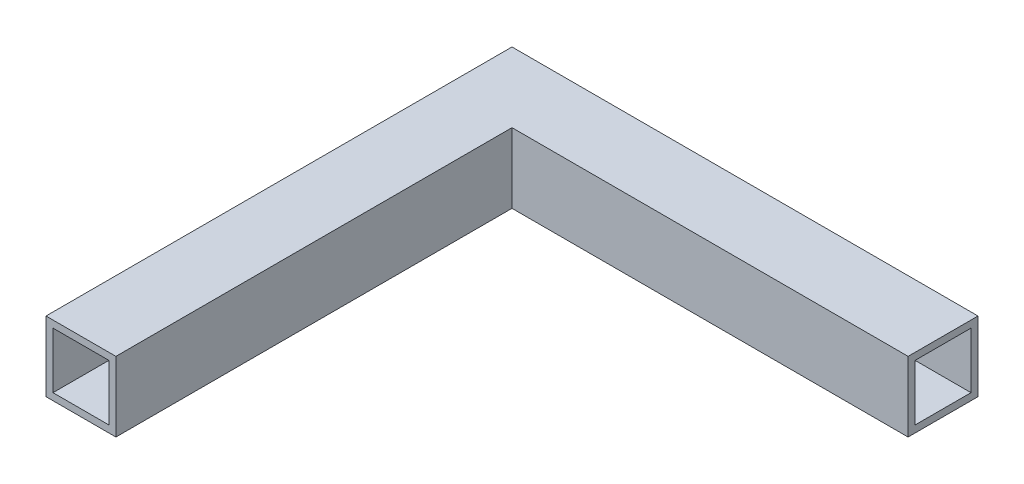
from build123d import *

# Parameters (mm, degrees)
SKETCH_1_W      = 200
SKETCH_1_H      = 30
EXTRUDE_1_DEPTH = 30
SKETCH_2_W      = 30
SKETCH_2_H      = 30
EXTRUDE_2_DEPTH = 170
SHELL_1_T       = -3


with BuildPart() as part:
    # 草图1 → 凸台-拉伸1 (new body)
    with BuildSketch(Plane.XY):
        with Locations((100, 15)):
            Rectangle(SKETCH_1_W, SKETCH_1_H)
    extrude(amount=-EXTRUDE_1_DEPTH)

    # 草图2 → 凸台-拉伸2 (add)
    with BuildSketch(Plane.XY):
        with Locations((15, 15)):
            Rectangle(SKETCH_2_W, SKETCH_2_H)
    extrude(amount=EXTRUDE_2_DEPTH)

    # 抽壳1
    shell_1_openings = [part.faces().sort_by_distance(p)[0] for p in [
        (15, 15, 170),
        (200, 15, -15),
    ]]
    offset(amount=SHELL_1_T, openings=shell_1_openings, kind=Kind.INTERSECTION)


solid = part.part
